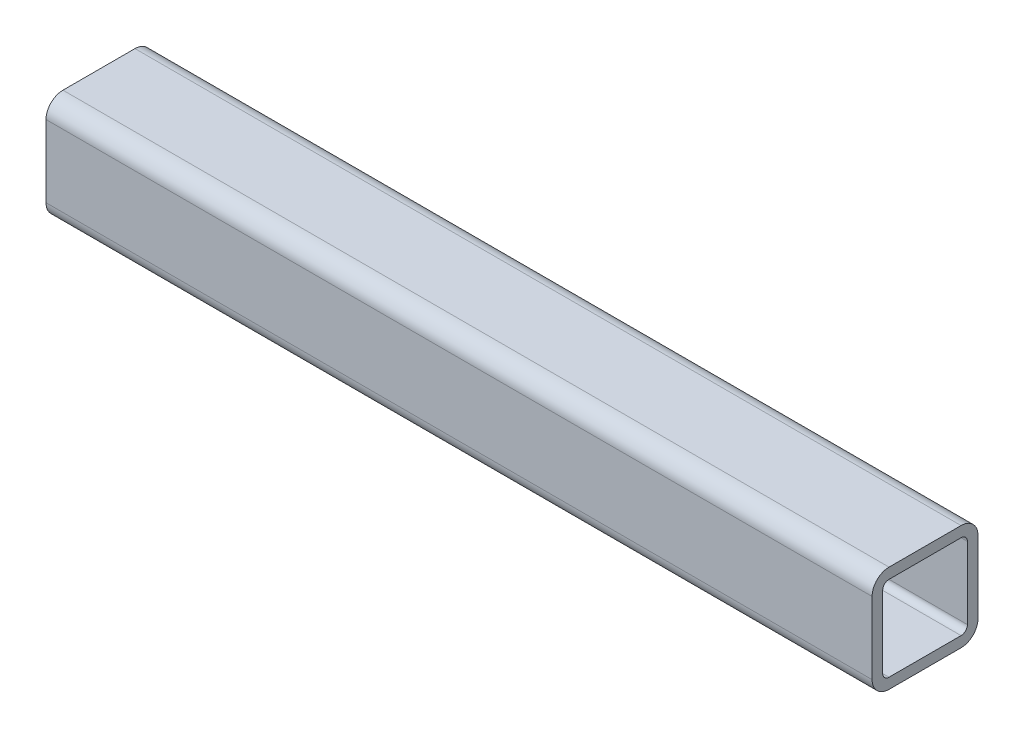
SolidWorks part; units mm, degrees
ref_plane "Front Plane" through (0, 0, 0) normal (0, 0, 1) x (1, 0, 0)
ref_plane "Top Plane" through (0, 0, 0) normal (0, 1, 0) x (1, 0, 0)
ref_plane "Right Plane" through (0, 0, 0) normal (1, 0, 0) x (0, 0, -1)
sketch "草图1" plane through (0, 0, 0) normal (0, 0, 1) x (1, 0, 0)
  line L0 (-88.4341, 0) -> (301.5659, 0)
  dimension "D1" = 390
other "Cold-formed square hollow section GB/T 6728-2002 50 X 50 X 4(1)"
ref_plane "Plane1" through (-88.4341, 0, 0) normal (1, 0, 0) x (0, 1, 0)
sketch "Sketch1" plane through (-88.4341, 0, 0) normal (1, 0, 0) x (0, 1, 0)
  line L0 (-17, -20) -> (17, -20)
  line L1 (-20, -17) -> (-20, 17)
  line L2 (17, 20) -> (-17, 20)
  line L3 (20, 17) -> (20, -17)
  line L4 (-17, -25) -> (17, -25)
  line L5 (-25, -17) -> (-25, 17)
  line L6 (17, 25) -> (-17, 25)
  line L7 (25, 17) -> (25, -17)
  arc A0 (25, 17) -> (17, 25) centre (17, 17) ccw
  arc A1 (17, -25) -> (25, -17) centre (17, -17) ccw
  arc A2 (-25, -17) -> (-17, -25) centre (-17, -17) ccw
  arc A3 (-17, 25) -> (-25, 17) centre (-17, 17) ccw
  arc A4 (-17, 20) -> (-20, 17) centre (-17, 17) ccw
  arc A5 (20, 17) -> (17, 20) centre (17, 17) ccw
  arc A6 (17, -20) -> (20, -17) centre (17, -17) ccw
  arc A7 (-20, -17) -> (-17, -20) centre (-17, -17) ccw
  point P0 (-25, 0)
  point P1 (25, 0)
  point P2 (0, 25)
  point P3 (0, -25)
  point P4 (0, 0)
  point P5 (-25, -25)
  point P6 (25, -25)
  point P7 (25, 25)
  point P8 (-25, 25)
  point P33 (0, 0)
  dimension "D1" = 8
  dimension "Thickness" = 5
  dimension "V_leg" = 50
